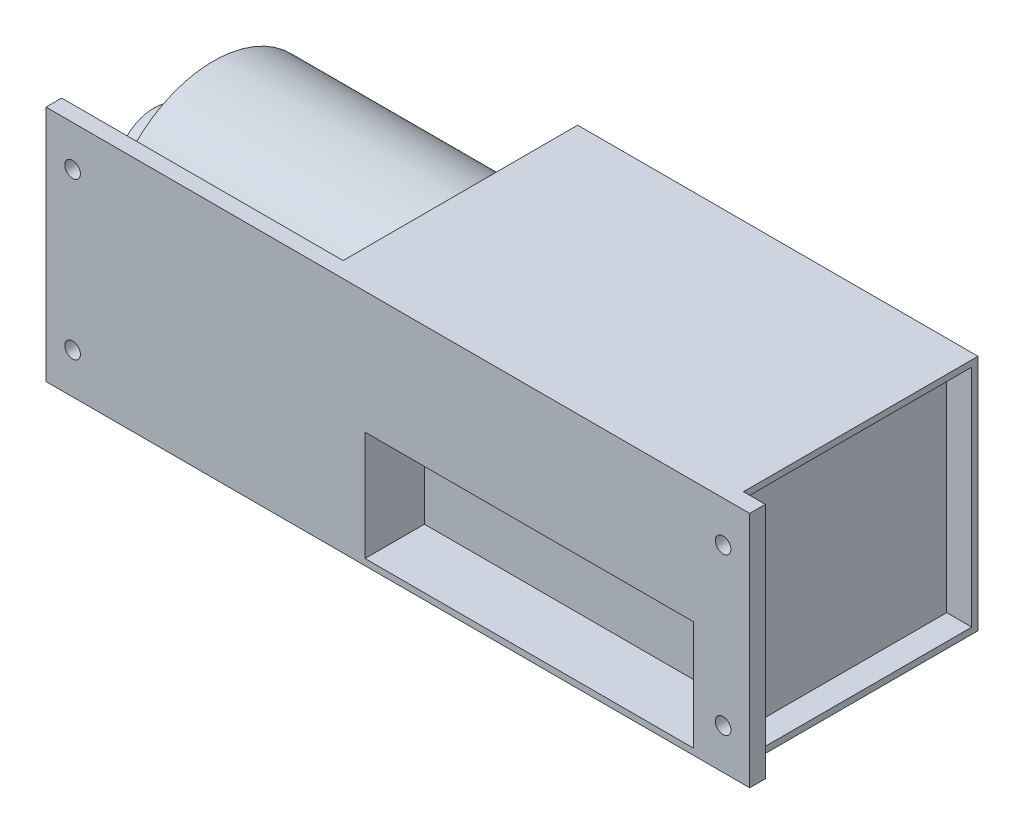
SolidWorks part; units mm, degrees
material "普通碳钢"
ref_plane "前视基准面" through (0, 0, 0) normal (0, 0, 1) x (1, 0, 0)
ref_plane "上视基准面" through (0, 0, 0) normal (0, 1, 0) x (1, 0, 0)
ref_plane "右视基准面" through (0, 0, 0) normal (1, 0, 0) x (0, 0, -1)
sketch "草图1" plane through (0, 0, 0) normal (0, 0, 1) x (1, 0, 0)
  line L1 (-112.5, 38) -> (112.5, 38)
  line L2 (-112.5, 38) -> (-112.5, -38)
  line L3 (-112.5, -38) -> (112.5, -38)
  line L4 (112.5, 38) -> (112.5, -38)
  line L5 (-112.5, 38) -> (112.5, -38) construction
  line L6 (-112.5, -38) -> (112.5, 38) construction
  point P0 (0, 0)
  dimension "D1" = 225
  dimension "D2" = 76
extrude "凸台-拉伸1" add sketch "草图1" along normal blind 80
sketch "草图2" plane through (-112.5, 0, 0) normal (-1, 0, 0) x (0, 0, 1)
  line L0 (80, 38) -> (0, 38) construction
  line L1 (0, -38) -> (75, -38)
  line L2 (0, -38) -> (0, 38)
  line L3 (0, 38) -> (75, 38)
  line L4 (75, -38) -> (75, 38)
  line L5 (80, 38) -> (80, -38) construction
  dimension "D1" = 5
extrude "切除-拉伸1" cut sketch "草图2" against normal blind 90
sketch "草图3" plane through (112.5, 0, 0) normal (1, 0, 0) x (0, 0, -1)
  line L0 (-80, -38) -> (0, -38) construction
  line L1 (0, 38) -> (-75, 38)
  line L2 (0, 38) -> (0, -38)
  line L3 (0, -38) -> (-75, -38)
  line L4 (-75, 38) -> (-75, -38)
  line L5 (-80, -38) -> (-80, 38) construction
  dimension "D1" = 5
extrude "切除-拉伸2" cut sketch "草图3" against normal blind 15
sketch "草图4" plane through (0, 0, 75) normal (0, 0, -1) x (-1, 0, 0)
  line L1 (104, -25) -> (-104, -25) construction
  line L2 (104, -25) -> (104, 25) construction
  line L3 (104, 25) -> (-104, 25) construction
  line L4 (-104, -25) -> (-104, 25) construction
  line L5 (104, -25) -> (-104, 25) construction
  line L6 (104, 25) -> (-104, -25) construction
  circle A0 centre (104, -25) radius 2.5
  circle A1 centre (104, 25) radius 2.5
  circle A2 centre (-104, -25) radius 2.5
  circle A3 centre (-104, 25) radius 2.5
  point P0 (0, 0)
  dimension "D1" = 5
  dimension "D2" = 208
  dimension "D3" = 50
extrude "切除-拉伸3" cut sketch "草图4" against normal blind 15
sketch "草图5" plane through (-22.5, 0, 0) normal (-1, 0, 0) x (0, 0, 1)
  line L0 (0, 0) -> (75, 0) construction
  line L1 (75, -38) -> (75, 38) construction
  circle A0 centre (37.5, 0) radius 35
  dimension "D1" = 70
extrude "凸台-拉伸2" add sketch "草图5" along normal blind 79
sketch "草图6" plane through (-101.5, 0, 0) normal (-1, 0, 0) x (0, 0, 1)
  circle A0 centre (37.5, 0) radius 12.5
  dimension "D1" = 25
extrude "凸台-拉伸3" add sketch "草图6" along normal blind 19
sketch "草图7" plane through (0, 0, 80) normal (0, 0, 1) x (1, 0, 0)
  line L0 (112.5, -38) -> (112.5, 38) construction
  line L1 (-10.5, -1) -> (94.5, -1)
  line L2 (-10.5, -1) -> (-10.5, -36)
  line L3 (-10.5, -36) -> (94.5, -36)
  line L4 (94.5, -1) -> (94.5, -36)
  line L5 (-112.5, -38) -> (112.5, -38) construction
  dimension "D1" = 105
  dimension "D2" = 35
  dimension "D3" = 18
  dimension "D4" = 2
extrude "切除-拉伸4" cut sketch "草图7" against normal blind 19
sketch "草图8" plane through (97.5, 0, 0) normal (1, 0, 0) x (0, 0, -1)
  line L0 (-75, 38) -> (0, 38)
  line L1 (0, 38) -> (0, -38)
  line L2 (0, -38) -> (0, 38) construction
  line L3 (0, -38) -> (-75, -38)
  line L4 (-75, -38) -> (-75, -36)
  line L5 (-75, 38) -> (-75, -38) construction
  line L6 (0, 0) -> (-32.8836, 0) construction
  line L7 (-75, -36) -> (-2, -36)
  line L8 (-75, 36) -> (-2, 36)
  line L9 (-75, 38) -> (-75, 36)
  line L10 (-2, 36) -> (-2, -36)
  point P19 (-8.4693, -33.8335)
  dimension "D1" = 2
  dimension "D2" = 2
extrude "凸台-拉伸4" add sketch "草图8" along normal blind 8
